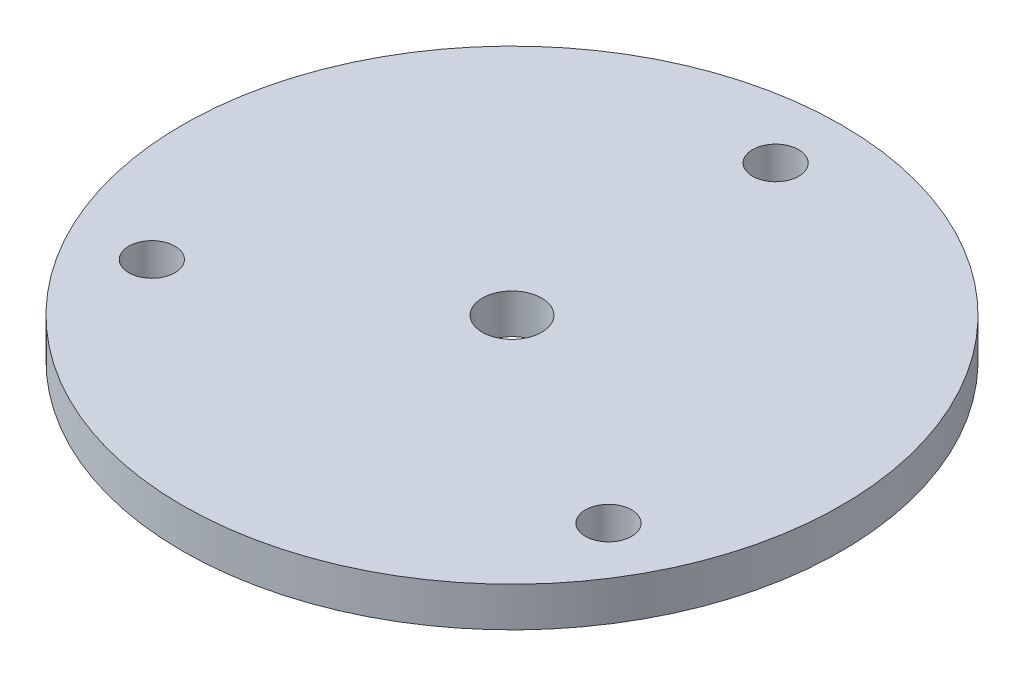
from build123d import *

# Parameters (mm, degrees)
SKETCH1_R              = 50
BOSS_EXTRUDE1_DEPTH    = 3
SKETCH2_R              = 3.5
CUT_EXTRUDE1_DEPTH     = 71.964779997
M10X1_0_TAPPED_HOLE1_D = 9


with BuildPart() as part:
    # Sketch1 → Boss-Extrude1 (new, symmetric)
    with BuildSketch(Plane(origin=(0, 0, 0), x_dir=(1, 0, 0), z_dir=(0, 1, 0))):
        with Locations(Location((0, 0, 0), (0, 0, 270))):
            Circle(SKETCH1_R)
    extrude(amount=BOSS_EXTRUDE1_DEPTH, both=True)

    # Sketch2 → Cut-Extrude1 (cut, through all)
    with BuildSketch(Plane(origin=(0, 3, 0), x_dir=(1, 0, 0), z_dir=(0, 1, 0))):
        with Locations(Location((0, 40, 0), (0, 0, 270))):
            Circle(SKETCH2_R)
        with Locations(Location((34.641016151, -20, 0), (0, 0, 270))):
            Circle(SKETCH2_R)
        with Locations(Location((-34.641016151, -20, 0), (0, 0, 270))):
            Circle(SKETCH2_R)
    extrude(amount=-CUT_EXTRUDE1_DEPTH, mode=Mode.SUBTRACT)

    # M10x1.0 Tapped Hole1 (through all)
    with Locations(Plane(origin=(0, 3, 0), x_dir=(1, 0, 0), z_dir=(0, 1, 0))):
        with Locations((0, 0)):
            Hole(M10X1_0_TAPPED_HOLE1_D / 2)


solid = part.part
